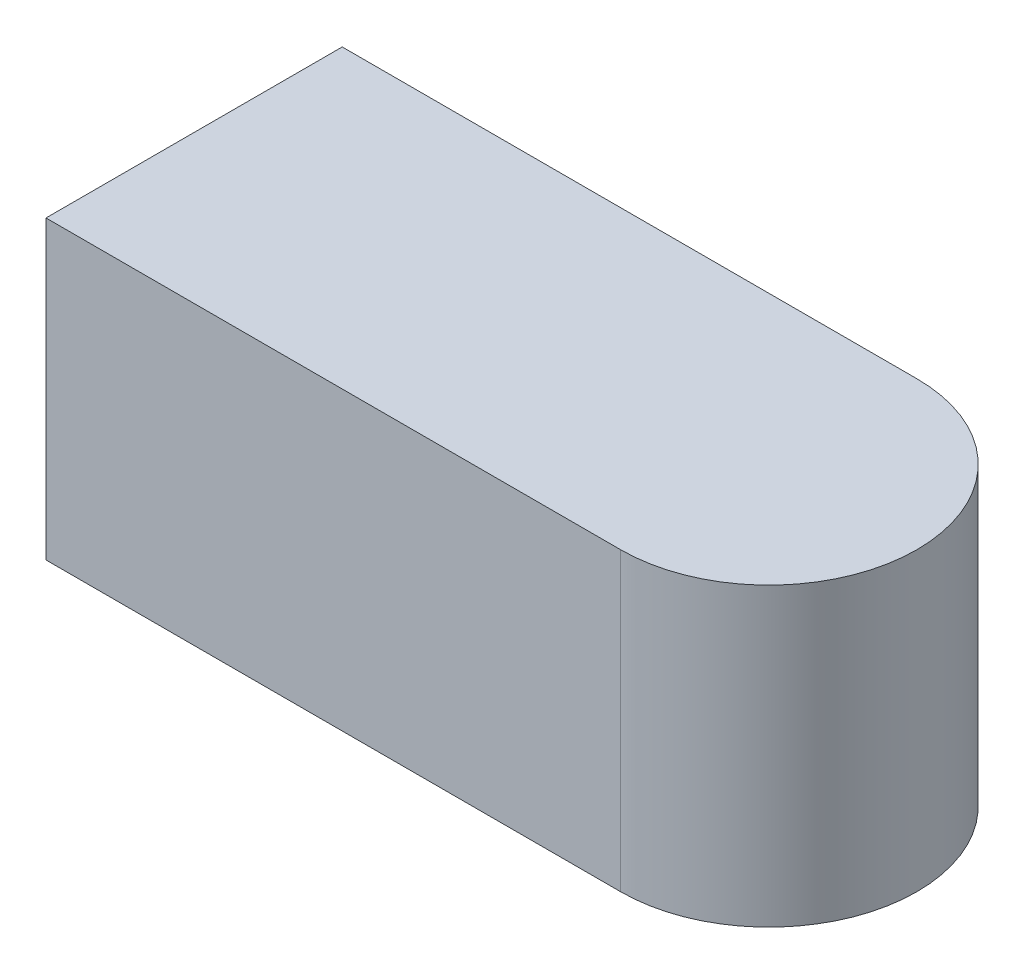
from build123d import *

# Parameters (mm, degrees)
BOSS_EXTRUDE1_DEPTH = 3.175
SKETCH2_R           = 2.4384
CUT_EXTRUDE1_DEPTH  = 11.1125


with BuildPart() as part:
    # Sketch1 → Boss-Extrude1 (new, symmetric)
    with BuildSketch(Plane(origin=(0, 0, 0), x_dir=(1, 0, 0), z_dir=(0, 1, 0))):
        with BuildLine():
            Line((0, 3.175), (12.319, 3.175))
            ThreePointArc((12.319, 3.175), (15.494, 0), (12.319, -3.175))
            Line((12.319, -3.175), (0, -3.175))
            Line((0, -3.175), (0, 3.175))
        make_face()
    extrude(amount=BOSS_EXTRUDE1_DEPTH, both=True)

    # Sketch2 → Cut-Extrude1 (cut)
    with BuildSketch(Plane.ZY):
        Circle(SKETCH2_R)
    extrude(amount=-CUT_EXTRUDE1_DEPTH, mode=Mode.SUBTRACT)

    # Sketch3 → Cut-Revolve1 (revolve, cut)
    with BuildSketch(Plane(origin=(0, 0, 0), x_dir=(1, 0, 0), z_dir=(0, 1, 0))):
        Polygon((13.917558324, 0), (11.1125, -2.4384), (0, -2.4384), (0, 0), align=None)
    revolve(axis=Axis((0, 0, 0), (1, 0, 0)), mode=Mode.SUBTRACT)


solid = part.part
